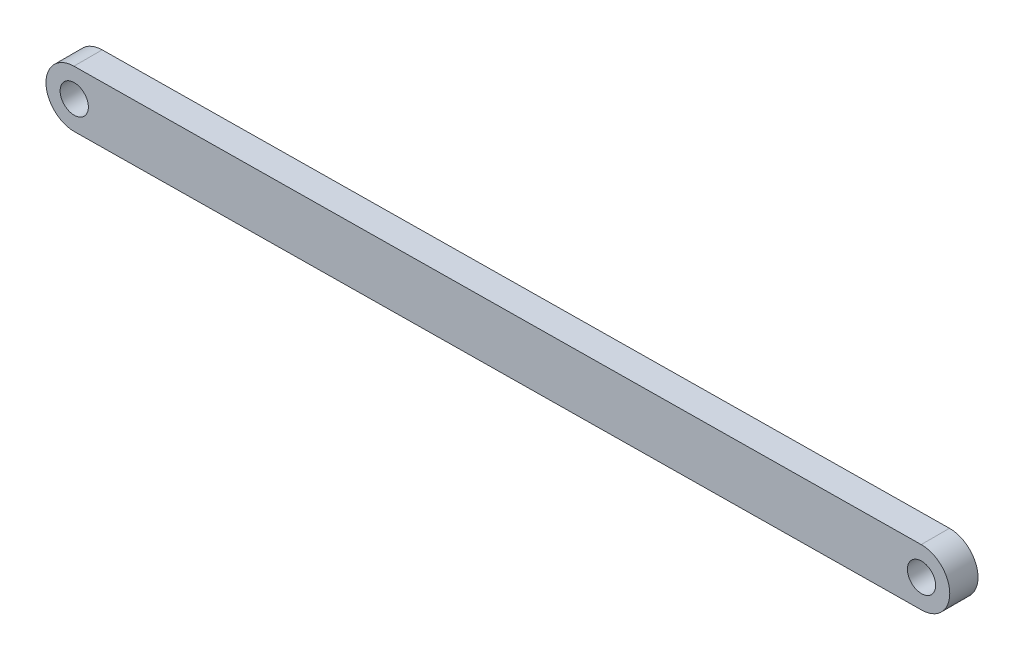
SolidWorks part; units mm, degrees
material "普通碳钢"
ref_plane "Front Plane" through (0, 0, 0) normal (0, 0, 1) x (1, 0, 0)
ref_plane "Top Plane" through (0, 0, 0) normal (0, 1, 0) x (1, 0, 0)
ref_plane "Right Plane" through (0, 0, 0) normal (1, 0, 0) x (0, 0, -1)
sketch "Sketch1" plane through (0, 0, 0) normal (0, 0, 1) x (1, 0, 0)
  line L0 (-0.1099, 9.9994) -> (299.872, 13.295)
  line L1 (0.1099, -9.9994) -> (300.0918, -6.7038)
  arc A0 (-0.1099, 9.9994) -> (0.1099, -9.9994) centre (0, 0) ccw
  arc A1 (300.0918, -6.7038) -> (299.872, 13.295) centre (299.9819, 3.2956) ccw
  circle A2 centre (299.9819, 3.2956) radius 5
  circle A3 centre (0, 0) radius 5
  dimension "D3" = 300
  dimension "D1" = 20
  dimension "D2" = 10
extrude "Boss-Extrude1" add sketch "Sketch1" along normal blind 10
